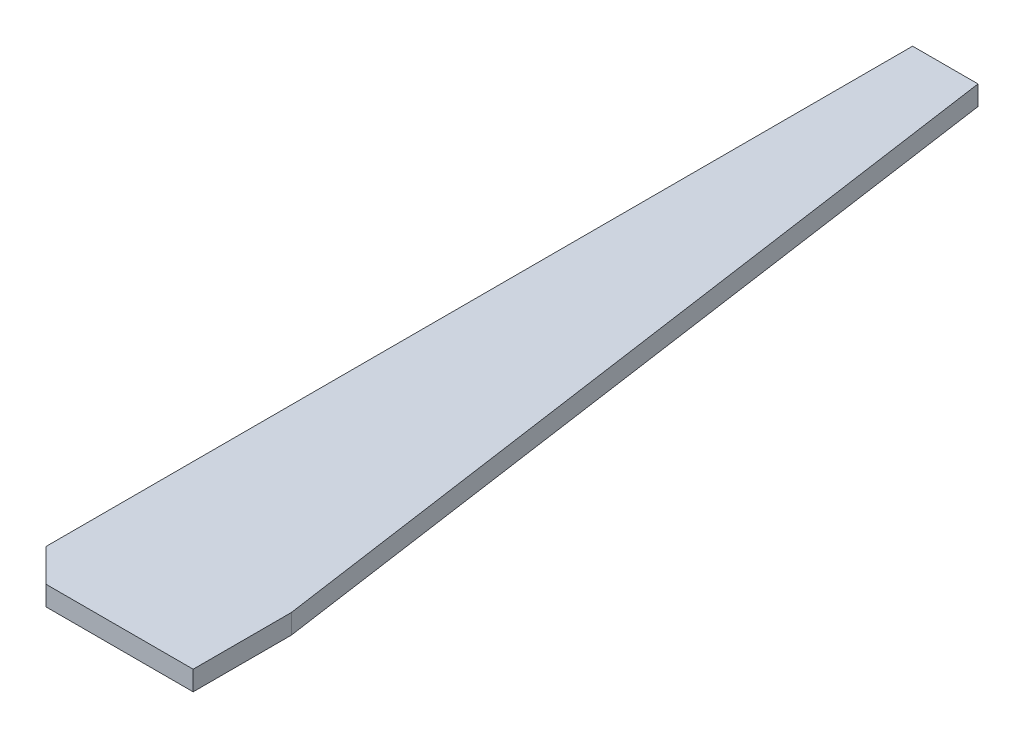
from build123d import *

# Parameters (mm, degrees)
BOSS_EXTRUDE1_DEPTH = 6
CHAMFER1_SIZE       = 20


with BuildPart() as part:
    # Sketch1 → Boss-Extrude1 (new, symmetric)
    with BuildSketch(Plane(origin=(0, 0, 0), x_dir=(1, 0, 0), z_dir=(0, 1, 0))):
        Polygon((-20, 20), (-20, 550), (20, 550), (90, 60), (90, 0), (0, 0), (-20, 0), align=None)
    extrude(amount=BOSS_EXTRUDE1_DEPTH, both=True)

    # Chamfer1
    chamfer1_edges = [part.edges().sort_by_distance(p)[0] for p in [
        (-20, 0, 0),
    ]]
    chamfer(chamfer1_edges, length=CHAMFER1_SIZE)


solid = part.part
